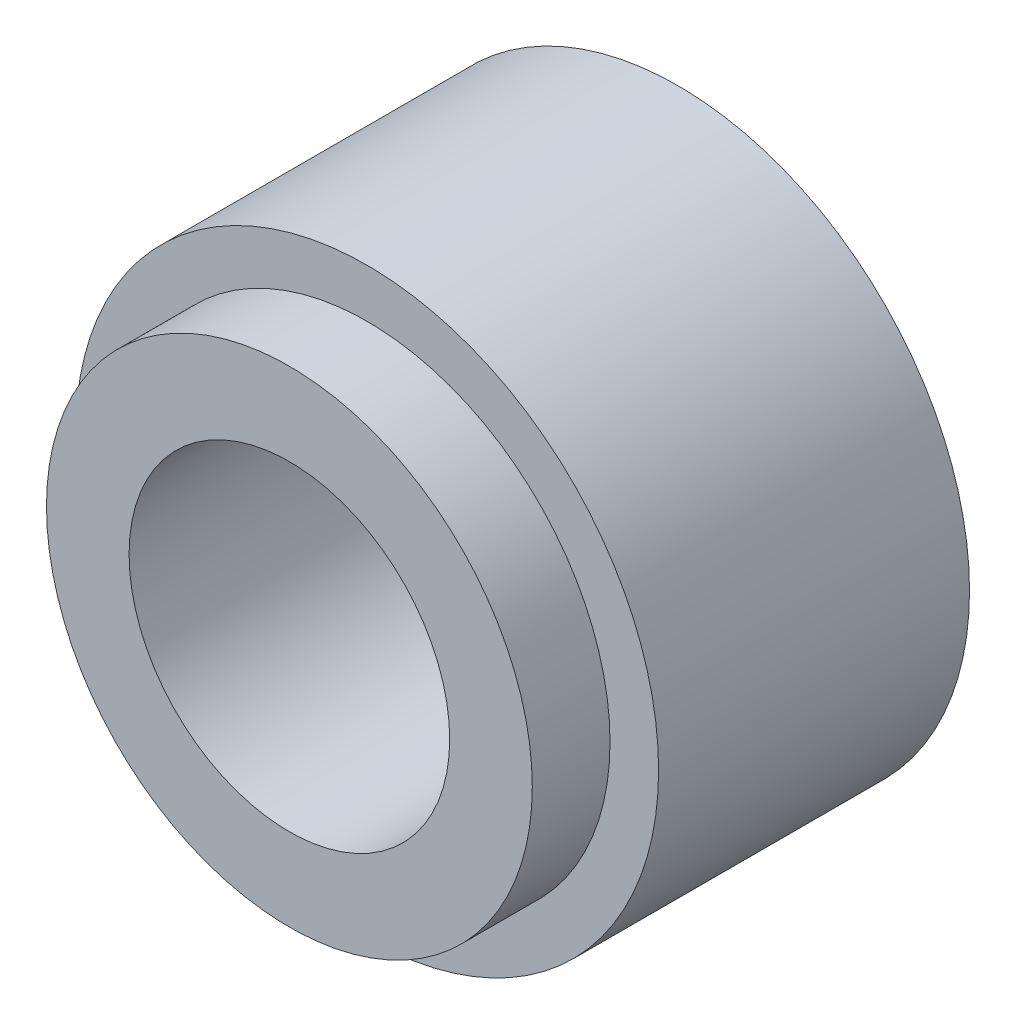
from build123d import *

# Parameters (mm, degrees)
M18X1_5_TAPPED_HOLE1_D     = 16.5
M18X1_5_TAPPED_HOLE1_DEPTH = 43.5
M18X1_5_TAPPED_HOLE1_TIP   = 4.957100107
CHAMFER1_SIZE              = 0.75


with BuildPart() as part:
    # Sketch1 → Revolve1 (revolve)
    with BuildSketch(Plane(origin=(0, 0, 0), x_dir=(1, 0, 0), z_dir=(0, 1, 0))):
        Polygon((7.5, 0), (12.5, 0), (12.5, 4), (15, 4), (15, 20), (7.5, 20), align=None)
    revolve(axis=Axis((0, 0, 0), (0, 0, -1)))

    # M18x1.5 Tapped Hole1
    with Locations(Plane(origin=(0, 0, -20), x_dir=(-1, 0, 0), z_dir=(0, 0, -1))):
        with Locations((0, 0)):
            Hole(M18X1_5_TAPPED_HOLE1_D / 2, depth=M18X1_5_TAPPED_HOLE1_DEPTH)
            with Locations((0, 0, -(M18X1_5_TAPPED_HOLE1_DEPTH + M18X1_5_TAPPED_HOLE1_TIP / 2))):  # 118° drill point
                Cone(0, M18X1_5_TAPPED_HOLE1_D / 2, M18X1_5_TAPPED_HOLE1_TIP, mode=Mode.SUBTRACT)

    # Chamfer1
    chamfer1_edges = [part.edges().sort_by_distance(p)[0] for p in [
        (-8.25, 0, -20),
    ]]
    chamfer(chamfer1_edges, length=CHAMFER1_SIZE)


solid = part.part
